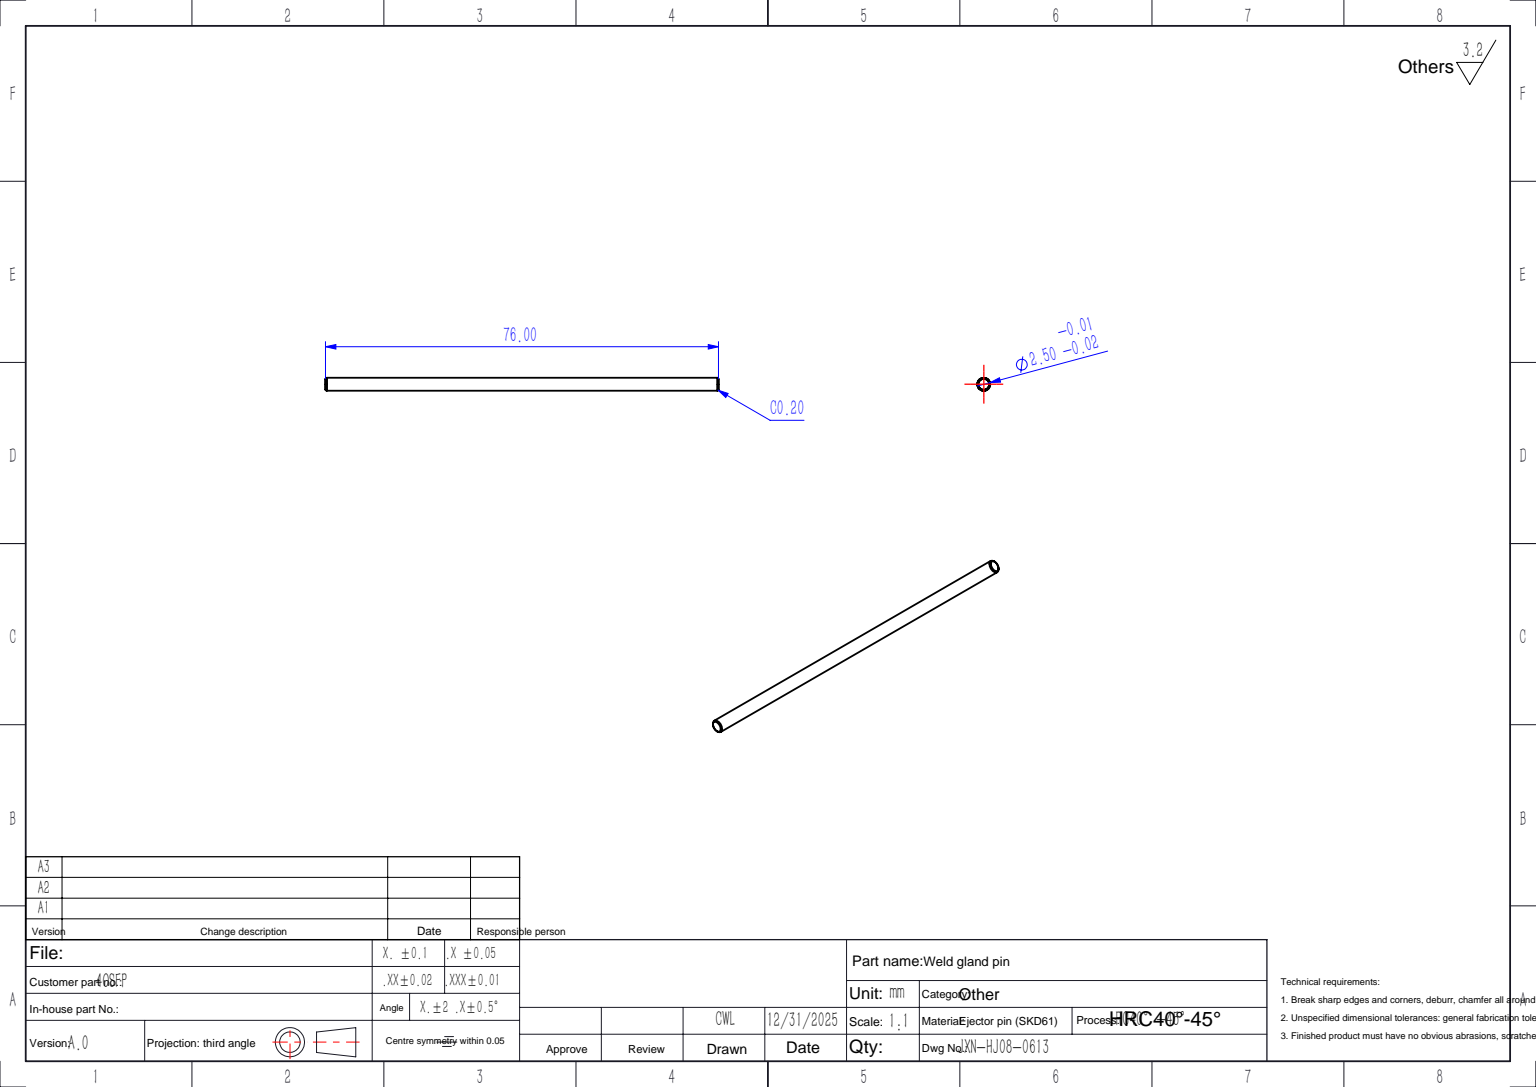
SolidWorks part; units mm, degrees
material "SKD61"
ref_plane "前视基准面" through (0, 0, 0) normal (0, 0, 1) x (1, 0, 0)
ref_plane "上视基准面" through (0, 0, 0) normal (0, 1, 0) x (1, 0, 0)
ref_plane "右视基准面" through (0, 0, 0) normal (1, 0, 0) x (0, 0, -1)
sketch "草图1" plane through (0, 0, 0) normal (0, 1, 0) x (1, 0, 0)
  circle A0 centre (0, 0) radius 1.25
  dimension "D1" = 2.5
extrude "凸台-拉伸1" add sketch "草图1" along normal blind 76
chamfer "倒角1" distance 0.2 angle 45 2 edges at (0, 76, 1.25) (0, 0, 1.25)
equation "\"code1\"= \"图名分离代码\""
equation "\"code2\"= \"图号分离代码\""
